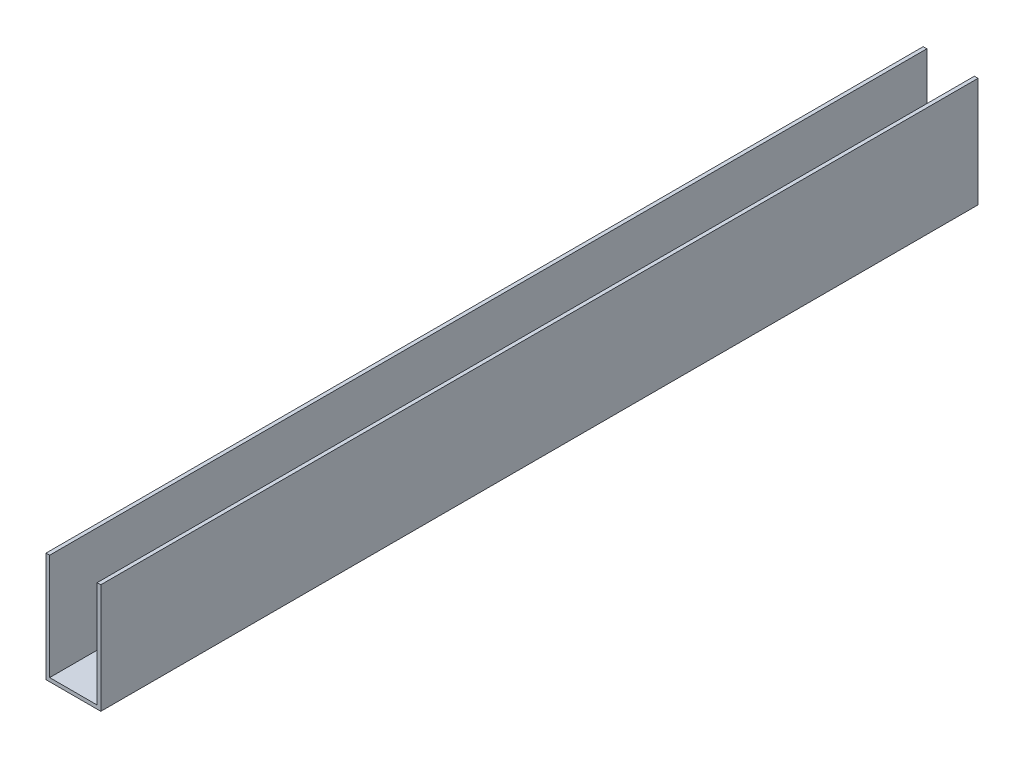
from build123d import *

# Parameters (mm, degrees)
SKETCH_1_W      = 30
SKETCH_1_H      = 60
EXTRUDE_1_DEPTH = 240
SHELL_1_T       = -2


with BuildPart() as part:
    # 草图1 → 凸台-拉伸1 (new, symmetric)
    with BuildSketch(Plane.XY):
        Rectangle(SKETCH_1_W, SKETCH_1_H)
    extrude(amount=EXTRUDE_1_DEPTH, both=True)

    # 抽壳1
    shell_1_openings = [part.faces().sort_by_distance(p)[0] for p in [
        (0, 0, 240),
        (0, 0, -240),
        (0, 30, 0),
    ]]
    offset(amount=SHELL_1_T, openings=shell_1_openings, kind=Kind.INTERSECTION)


solid = part.part
